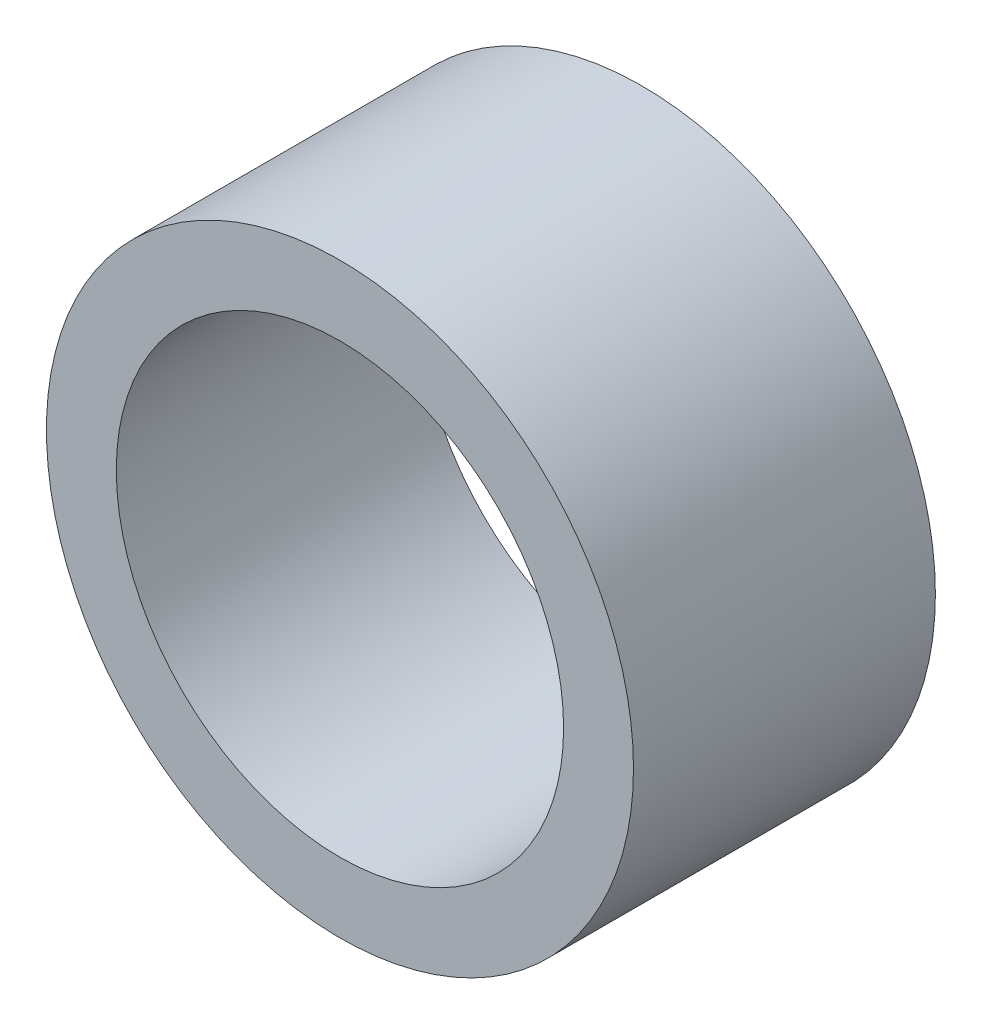
SolidWorks part; units mm, degrees
ref_plane "前视基准面" through (0, 0, 0) normal (0, 0, 1) x (1, 0, 0)
ref_plane "上视基准面" through (0, 0, 0) normal (0, 1, 0) x (1, 0, 0)
ref_plane "右视基准面" through (0, 0, 0) normal (1, 0, 0) x (0, 0, -1)
sketch "草图1" plane through (0, 0, 0) normal (0, 0, 1) x (1, 0, 0)
  circle A0 centre (0, 0) radius 210
extrude "凸台-拉伸1" add sketch "草图1" along normal blind 216
sketch "草图2" plane through (0, 0, 0) normal (0, 0, 1) x (1, 0, 0)
  circle A0 centre (0, 0) radius 160
extrude "切除-拉伸1" cut sketch "草图2" along normal blind 250
